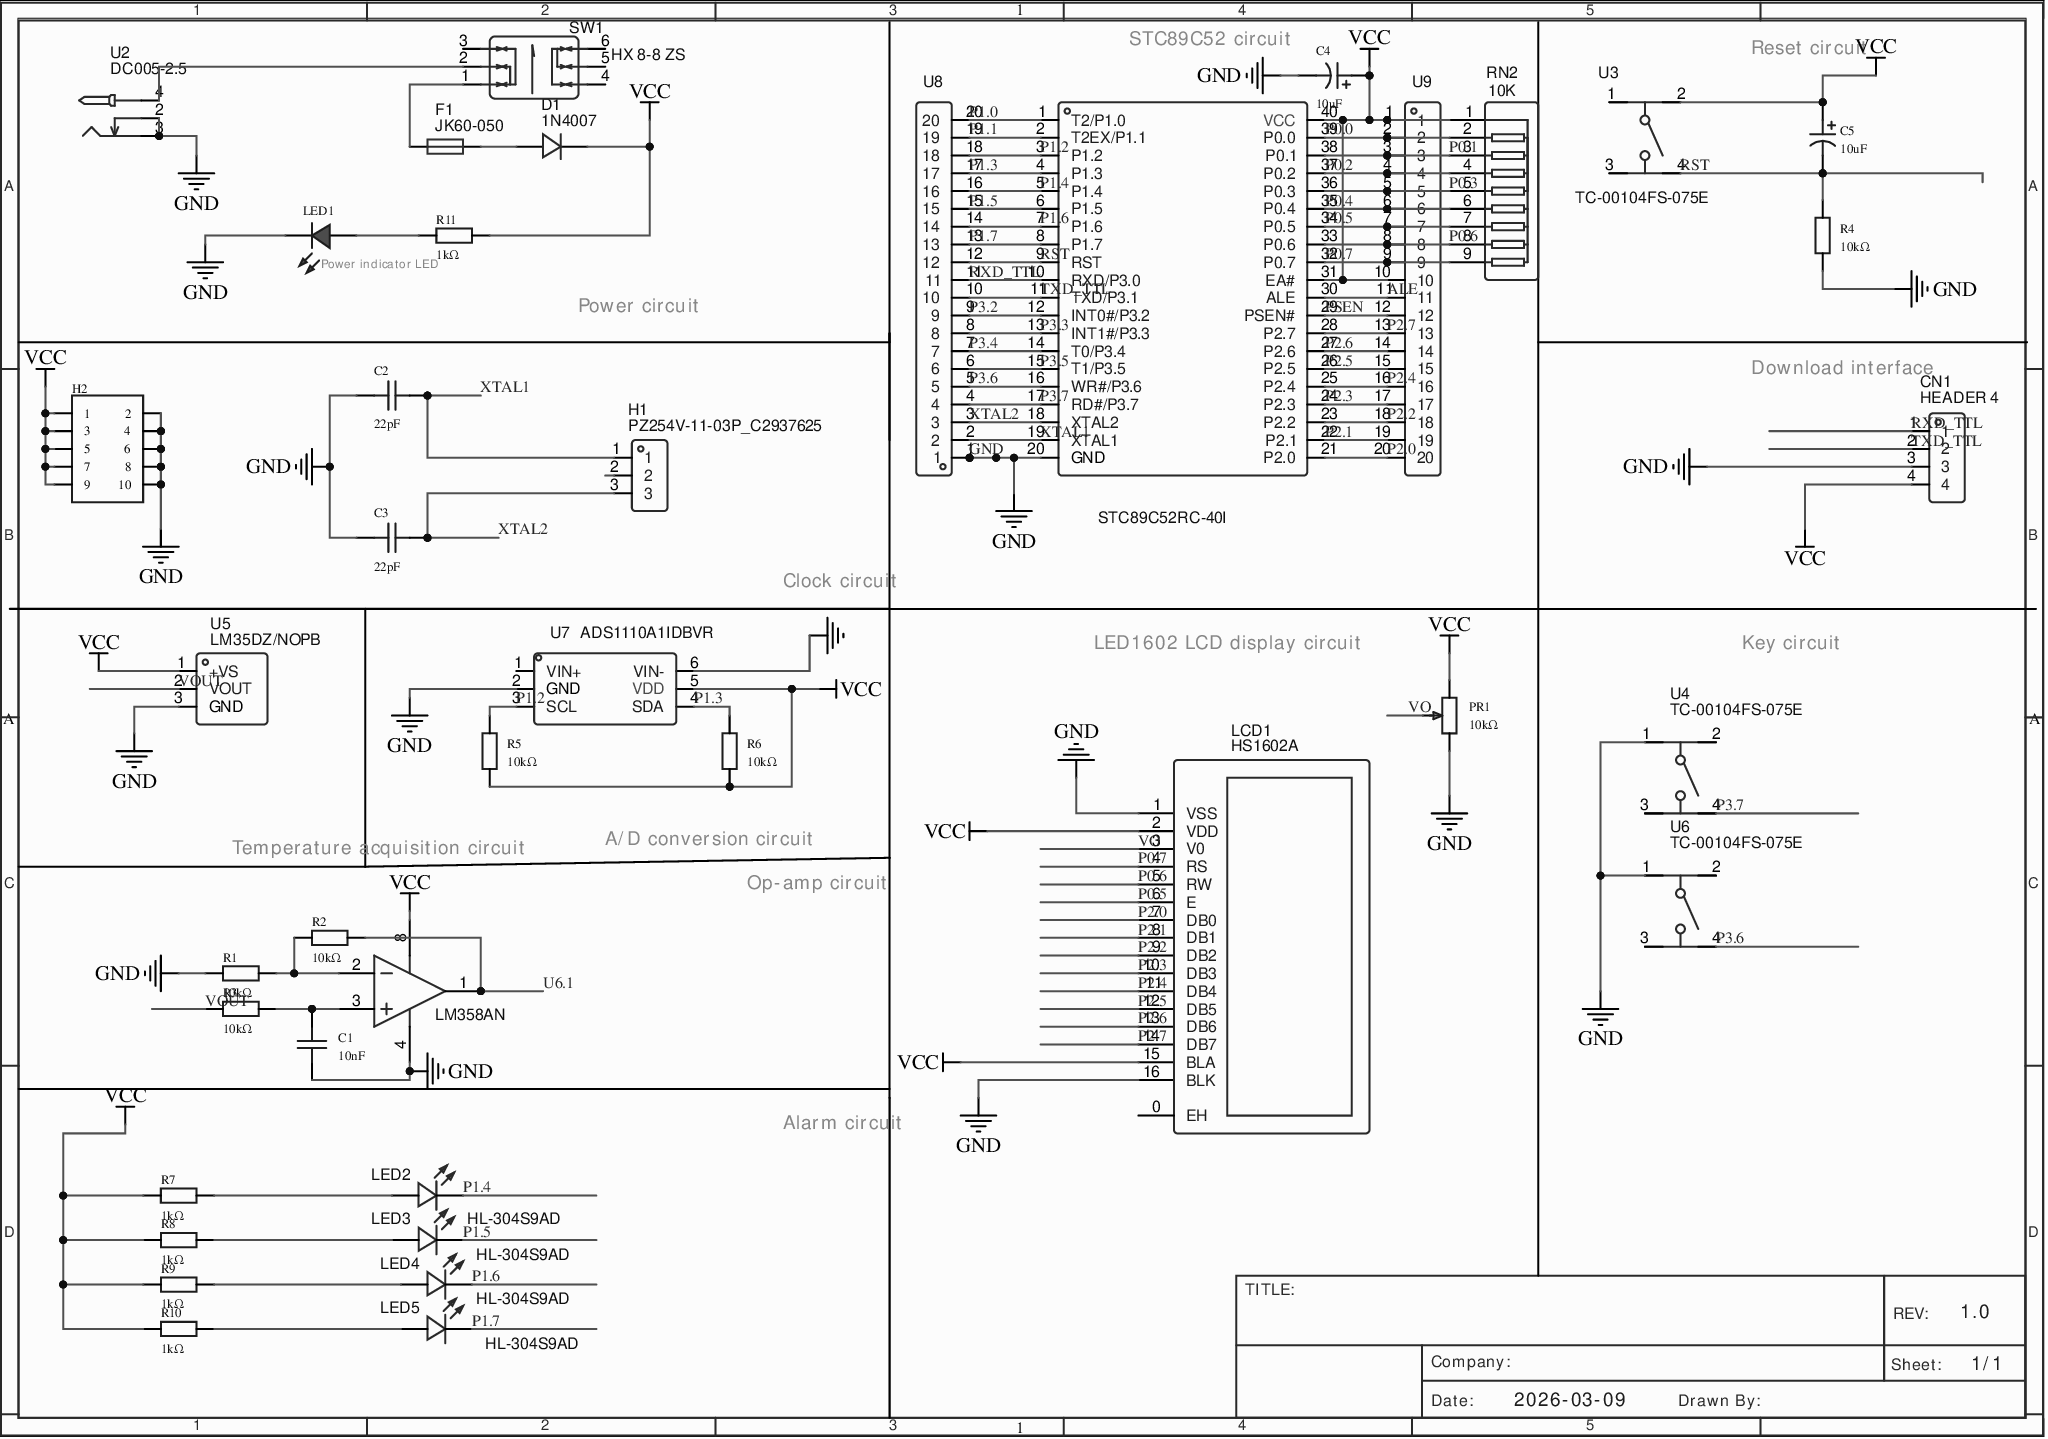
[diagram p0: MISC75226-3.schdoc]
# Altium project MISC75226-2.PrjPcb
1 sheet, 40 parts. Net scope: global (net labels, ports and power ports of the same name join across sheets).
Board file: MISC75226.pcbdoc

## Sheet MISC75226-3.schdoc
size 292 x 205 mm; Name: MISC75226; @Project Name: MISC75226; REV: 1.0; Date: 2026-03-09; Sheet: 1/1; Manufacturer Part: ?

### Parts
C1  10nF  [CAP-TH_L4.5-W2.5-P5.00-D0.5]
C2  22pF  [CAP-TH_L4.8-W3.2-P5.08-D0.5]
C3  22pF  [CAP-TH_L4.8-W3.2-P5.08-D0.5]
C4  10uF  [CAP-TH_BD5.0-P2.00-D0.8-FD-10UF50VC110GL]
C5  10uF  [CAP-TH_BD5.0-P2.00-D0.8-FD-10UF50VC110GL]
CN1  HEADER 4  [CONN-TH_XH-4A]
D1  1N4007  [DO-41_BD2.4-L4.7-P8.70-D0.9-RD]
F1  JK60-050  [FUSE-TH_L8.9-W3.0-P5.10-D0.6-S1.20]
H1  PZ254V-11-03P_C2937625  [HDR-TH_3P-P2.54-V-M_PZ254V-11-03P]
H2  (no value)  [HDR-TH_10P-P2.54-V-F-R2-C5-S2.54]
LCD1  HS1602A  [LCD1602]
LED1  (no value)  [LED_TH-3mm]
LED2  HL-304S9AD  [LED-TH_BD3.0-P2.54-FD]
LED3  HL-304S9AD  [LED-TH_BD3.0-P2.54-FD]
LED4  HL-304S9AD  [LED-TH_BD3.0-P2.54-FD]
LED5  HL-304S9AD  [LED-TH_BD3.0-P2.54-FD]
PR1  10kΩ  [R_3296]
R1  10kΩ  [Res_1/8W]
R2  10kΩ  [Res_1/8W]
R3  10kΩ  [Res_1/8W]
R4  10kΩ  [Res_1/8W]
R5  10kΩ  [Res_1/8W]
R6  10kΩ  [Res_1/8W]
R7  1kΩ  [Res_1/8W]
R8  1kΩ  [Res_1/8W]
R9  1kΩ  [Res_1/8W]
R10  1kΩ  [Res_1/8W]
R11  1kΩ  [Res_1/8W]
RN2  10K  [RES-ARRAY-TH_9P-P2.54-D1.0]
SW1  HX 8-8 ZS  [SW-TH_6P-L8.0-W8.0-P2.50-TL]
U1  LM358AN  [DIP-8_L9.8-W6.6-P2.54-LS7.6-BL]
U2  DC005-2.5  [DC-IN-TH_DC005-2.5MM]
U3  TC-00104FS-075E  [KEY-TH_4P-L6.0-W6.0-P4.50-LS6.5]
U4  TC-00104FS-075E  [KEY-TH_4P-L6.0-W6.0-P4.50-LS6.5]
U5  LM35DZ/NOPB  [TO-92-3_L4.8-W3.7-P2.54-L]
U6  TC-00104FS-075E  [KEY-TH_4P-L6.0-W6.0-P4.50-LS6.5]
U7  ADS1110A1IDBVR  [SOT-23-6_L2.9-W1.6-P0.95-LS2.8-BR]
U8  [Plugin] 2.54MM 1*20P straight female header-H5.0  [HDR-TH_20P-P2.54_C9900009338]  (value not drawn)
U9  [Plugin] 2.54MM 1*20P straight female header-H5.0  [HDR-TH_20P-P2.54_C9900009338]  (value not drawn)
U100  STC89C52RC-40I  [DIP-40_L52.0-W13.7-P2.54-LS15.2-BL]

### Nets
GND: C1.1 C2.1 C3.1 C4.2 CN1.3 H2.2 H2.4 H2.6 H2.8 H2.10 LCD1.1(VSS) LCD1.16(BLK) LED1.2(A) PR1.3 R1.1 R4.1 U1.4(GND) U2.2 U2.3 U4.1 U5.3(GND) U6.1 U7.2(GND) U7.6(VIN-) U8.1 U100.20(GND)
VCC: C4.1 C5.1 CN1.4 D1.1(K) H2.1 H2.3 H2.5 H2.7 H2.9 LCD1.2(VDD) LCD1.15(BLA) PR1.1 R5.1 R6.1 R7.1 R8.1 R9.1 R10.1 R11.2 RN2.1 U1.8(VCC) U3.2 U5.1(+VS) U7.5(VDD) U9.1 U9.10 U100.31(EA#) U100.40(VCC)
ALE: U9.11 U100.30(ALE)
P0.0: RN2.2 U9.2 U100.39(P0.0)
P0.1: RN2.3 U9.3 U100.38(P0.1)
P0.2: RN2.4 U9.4 U100.37(P0.2)
P0.3: RN2.5 U9.5 U100.36(P0.3)
P0.4: RN2.6 U9.6 U100.35(P0.4)
P0.5: LCD1.6(E) RN2.7 U9.7 U100.34(P0.5)
P0.6: LCD1.5(RW) RN2.8 U9.8 U100.33(P0.6)
P0.7: LCD1.4(RS) RN2.9 U9.9 U100.32(P0.7)
P1.0: U8.20 U100.1(T2/P1.0)
P1.1: U8.19 U100.2(T2EX/P1.1)
P1.2: R5.2 U7.3(SCL) U8.18 U100.3(P1.2)
P1.3: R6.2 U7.4(SDA) U8.17 U100.4(P1.3)
P1.4: LED2.2(C) U8.16 U100.5(P1.4)
P1.5: LED3.2(C) U8.15 U100.6(P1.5)
P1.6: LED4.2(C) U8.14 U100.7(P1.6)
P1.7: LED5.2(C) U8.13 U100.8(P1.7)
P2.0: LCD1.7(DB0) U9.20 U100.21(P2.0)
P2.1: LCD1.8(DB1) U9.19 U100.22(P2.1)
P2.2: LCD1.9(DB2) U9.18 U100.23(P2.2)
P2.3: LCD1.10(DB3) U9.17 U100.24(P2.3)
P2.4: LCD1.11(DB4) U9.16 U100.25(P2.4)
P2.5: LCD1.12(DB5) U9.15 U100.26(P2.5)
P2.6: LCD1.13(DB6) U9.14 U100.27(P2.6)
P2.7: LCD1.14(DB7) U9.13 U100.28(P2.7)
P3.2: U8.9 U100.12(INT0#/P3.2)
P3.3: U8.8 U100.13(INT1#/P3.3)
P3.4: U8.7 U100.14(T0/P3.4)
P3.5: U8.6 U100.15(T1/P3.5)
P3.6: U6.4 U8.5 U100.16(WR#/P3.6)
P3.7: U4.4 U8.4 U100.17(RD#/P3.7)
PSEN: U9.12 U100.29(PSEN#)
RST: C5.2 R4.2 U3.4 U8.12 U100.9(RST)
RXD_TTL: CN1.1 U8.11 U100.10(RXD/P3.0)
TXD_TTL: CN1.2 U8.10 U100.11(TXD/P3.1)
U6.1: R2.2 U1.1(OUT1)
VO: LCD1.3(V0) PR1.2
VOUT: R3.1 U5.2(VOUT)
XTAL1: C2.2 H1.1 U8.2 U100.19(XTAL1)
XTAL2: C3.2 H1.3 U8.3 U100.18(XTAL2)
NetC1_2: C1.2 R3.2 U1.3(IN1(+))
NetD1_2: D1.2(A) F1.2
NetF1_1: F1.1 SW1.1
NetLED1_1: LED1.1(C) R11.1
NetLED2_1: LED2.1(A) R7.2
NetLED3_1: LED3.1(A) R8.2
NetLED4_1: LED4.1(A) R9.2
NetLED5_1: LED5.1(A) R10.2
NetR1_2: R1.2 R2.1 U1.2(IN1(-))
NetSW1_2: SW1.2 U2.4

Not connected (* = marked no-connect by the designer): H1 2; LCD1 0(EH); SW1 3 4 5 6; U3 1 3; U4 2 3; U6 2 3; U7 1(VIN+)

### Notes on the sheet
- (near C4) STC89C52 circuit
- (near C5) Reset circuit
- Power indicator LED
- Power circuit
- (near CN1) Download interface
- Clock circuit
- LED1602 LCD display circuit
- Key circuit
- Temperature acquisition circuit
- (near R6) A/D conversion circuit
- Op-amp circuit
- Alarm circuit
- 1
- 2
- 3
- 4
- 5
- A
- B
- C
- D
- TITLE:
- Company:
- Sheet:
- REV:
- 1.0
- 1/1
- Date:
- 2026-03-09
- Drawn By:

### Library data of the parts
C1 = FK24C0G1H103JN006: 容值:10nF;精度:±5%;额定电压:50V;温度系数:C0G；NP0;; Manufacturer: TDK; AddInBom: yes; ModelId: a3610cc4d782423286e41c4ef8ce78f40819f05c4eef4c71ace90d822a990e87; ModelTransform: 216.535,98.8187,0,0,0,0,0,0,-196.85; Tolerance: ±5%; Voltage Rating: 50V; Temperature Coefficient: C0G; NP0; Symbol: FK24C0G1H103JN006; Device: FK24C0G1H103JN006; LCSC Part Name: 10nF ±5% 50V; SupplierPart: C5640246; ManufacturerPart: FK24C0G1H103JN006; Supplier Footprint: -; JLCPCB Part Class: Extended Part; Datasheet: https://item.szlcsc.com/datasheet/FK24C0G1H103JN006/6560964.html; Supplier: LCSC; ConvertToPcb: yes; FootprintName: CAP-TH_L4.5-W2.5-P5.00-D0.5; ModelName: CAP-TH_L4.5-W2.5-P5.00-D0.5; Value: 10nF
C2 C3 = CC4-0805-CG-50V-22pF-J: 容值:22pF;精度:±5%;额定电压:50V;温度系数:-;; Manufacturer: TORCH(火炬); AddInBom: yes; ModelId: f657e7819ee0481b9510acb89a450e410819f05c4eef4c71ace90d822a990e87; ModelName: CAP-TH_L4.8-W3.2-H6.8-P5.08; ModelTransform: 215.7476,125.984,0,0,0,0,0,0,-137.795; Tolerance: ±5%; Voltage Rating: 50V; Symbol: CC4-0805-CG -50V-22pF-J; Device: CC4-0805-CG-50V-22pF-J; LCSC Part Name: 22pF ±5% 50V; SupplierPart: C123150; ManufacturerPart: CC4-0805-CG-50V-22pF-J; Supplier Footprint: 插件,P=5.08mm; JLCPCB Part Class: Extended Part; Datasheet: https://item.szlcsc.com/datasheet/CC4-0805-CG-50V-22pF-J/124420.html; Supplier: LCSC; ConvertToPcb: yes; FootprintName: CAP-TH_L4.8-W3.2-P5.08-D0.5; Value: 22pF; Temperature Coefficient: -
C4 C5 = 10UF50VC110GL: 容值:10uF;精度:±20%;额定电压:50V;纹波电流:120mA@100KHz;等效串联电阻(ESR):1.6Ω;; Manufacturer: Econd(米朗电子); AddInBom: yes; Tolerance: ±20%; Voltage Rating: 50V; Equivalent Series Resistance(ESR): 1.6Ω; Pin Spacing: 2mm; Lifetime: 5000hrs@105℃; Symbol: 10UF50VC110GL; Device: 10UF50VC110GL; LCSC Part Name: 10uF ±20% 50V; SupplierPart: C46867109; ManufacturerPart: 10UF50VC110GL; Supplier Footprint: 插件,D5xL11mm; JLCPCB Part Class: Extended Part; Datasheet: https://item.szlcsc.com/datasheet/10UF50VC110GL/49031974.html; Supplier: LCSC; ConvertToPcb: yes; FootprintName: CAP-TH_BD5.0-P2.00-D0.8-FD-10UF50VC110GL; Value: 10uF; Ripple Current: 120mA@100KHz; Diameter: 5mm; Height - Seated (Max): 11mm; Operating Temperature: -40℃~+105℃
CN1 = Header 4: Manufacturer: null; Convert to PCB: yes; UniqueId: ggea3fdb8c5cd09fd78; ModelTransform: 492.125,228.346,0,0,0,0,-0.003,20.196,-129.921; Device: Header 4; Supplier: LCSC; Supplier Part: C9900017655; Manufacturer Part: Header 4; JLCPCB Part Class: Extended Part; Add into BOM: yes; SymbolName: HEADER 4; FootprintName: CONN-TH_XH-4A; OriginModelName: CONN-TH_XH-4A
D1 = 1N4007: Manufacturer: ST(先科); Convert to PCB: yes; UniqueId: ggea25f4b96c0c873f1; OriginModelName: DO-41_D2.4-L4.7-P8.70; ModelTransform: 374.016,94.488,0,0,0,0,0.002,0,-137.795; Device: 1N4007; Supplier: LCSC; Manufacturer Part: 1N4007; Supplier Part: C106903; JLCPCB Part Class: Extended Part; Add into BOM: yes; SymbolName: 1N4007; FootprintName: DO-41_BD2.4-L4.7-P8.70-D0.9-RD
F1 = JK60-050: Manufacturer: null; Convert to PCB: yes; UniqueId: gge1ed7edf1a1e32f02; OriginModelName: FUSE-TH_L8.9-W3.0-H13.5-P5.1-D0.6-S1.2; ModelTransform: 350.393,118.11,0,0,0,0,0,0,-275.591; Device: JK60-050; Supplier: LCSC; Supplier Part: C139092; Manufacturer Part: JK60-050; JLCPCB Part Class: Extended Part; Add into BOM: yes; SymbolName: JK60-050; FootprintName: FUSE-TH_L8.9-W3.0-P5.10-D0.6-S1.20
H1 = PZ254V-11-03P: Manufacturer: XFCN(兴飞); Convert to PCB: yes; UniqueId: ggee8450ff7c7c91b07; ModelTransform: 300.3931,100,0,0,0,0,-0.001,0.001,-118.11; Device: PZ254V-11-03P; Supplier: LCSC; Supplier Part: C2937625; Manufacturer Part: PZ254V-11-03P; JLCPCB Part Class: Extended Part; Add into BOM: yes; SymbolName: PZ254V-11-03P_C2937625; FootprintName: HDR-TH_3P-P2.54-V-M_PZ254V-11-03P; OriginModelName: HDR-TH_3P-P2.54-V-M_PZ254V-11-03P
H2 = HDR-F_2.54_2x5: Symbol: HDR-F-2.54_2x5; ConvertToPcb: yes; ModelId: 86e5d65f54dd476391caab3fdb9168240819f05c4eef4c71ace90d822a990e87; ModelName: HDR2.54-F-LI-2X5P; ModelTransform: 499.999,200,0,0,0,0,0,0,-118.11; Device: HDR-F_2.54_2x5; AddInBom: yes; SupplierPart: C92270; Supplier Footprint: 插件; FootprintName: HDR-TH_10P-P2.54-V-F-R2-C5-S2.54
LCD1 = HS1602A: Manufacturer: HS(汉昇); Convert to PCB: yes; UniqueId: gge471e28896b9a3d54; ModelTransform: 3149.6,1417.32,0,0,0,0,0,0,-118.11; Device: HS1602A; Supplier: LCSC; Supplier Part: C5329588; Manufacturer Part: HS1602A; JLCPCB Part Class: Extended Part; Add into BOM: yes; SymbolName: HS1602A; FootprintName: LCD1602; OriginModelName: LCD1602
LED1 = LED_TH-R_3mm: ConvertToPcb: yes; ModelId: a497c992633541038a38947cdc58012f0819f05c4eef4c71ace90d822a990e87; ModelName: LED-TH-3mm_R; ModelTransform: 141.274,153.327,0,0,0,0,-5.984,0,-137.795; Symbol: LED_TH-R; Device: LED_TH-R_3mm; AddInBom: yes; FootprintName: LED_TH-3mm; Supplier Footprint: 插件
LED2 = HL-304S9AD: Manufacturer: HONGLITRONIC(鸿利光电); Convert to PCB: yes; UniqueId: ggedcb368d0afbaf50c; OriginModelName: LED-TH-3mm_R; ModelTransform: 141.274,153.327,0,0,0,0,-5.983,0,-137.795; Device: HL-304S9AD; Supplier: LCSC; Supplier Part: C568936; Manufacturer Part: HL-304S9AD; JLCPCB Part Class: Extended Part; Add into BOM: yes; SymbolName: HL-304S9AD; FootprintName: LED-TH_BD3.0-P2.54-FD
LED3 = HL-304S9AD: Manufacturer: HONGLITRONIC(鸿利光电); Convert to PCB: yes; UniqueId: gge7e573e1ae17299c8; OriginModelName: LED-TH-3mm_R; ModelTransform: 141.274,153.327,0,0,0,0,-5.983,0,-137.795; Device: HL-304S9AD; Supplier: LCSC; Supplier Part: C568936; Manufacturer Part: HL-304S9AD; JLCPCB Part Class: Extended Part; Add into BOM: yes; SymbolName: HL-304S9AD; FootprintName: LED-TH_BD3.0-P2.54-FD
LED4 = HL-304S9AD: Manufacturer: HONGLITRONIC(鸿利光电); Convert to PCB: yes; UniqueId: gge9c2f58a485d7e2d3; OriginModelName: LED-TH-3mm_R; ModelTransform: 141.274,153.327,0,0,0,0,-5.983,0,-137.795; Device: HL-304S9AD; Supplier: LCSC; Supplier Part: C568936; Manufacturer Part: HL-304S9AD; JLCPCB Part Class: Extended Part; Add into BOM: yes; SymbolName: HL-304S9AD; FootprintName: LED-TH_BD3.0-P2.54-FD
LED5 = HL-304S9AD: Manufacturer: HONGLITRONIC(鸿利光电); Convert to PCB: yes; UniqueId: ggec88dd7fe630cf856; OriginModelName: LED-TH-3mm_R; ModelTransform: 141.274,153.327,0,0,0,0,-5.983,0,-137.795; Device: HL-304S9AD; Supplier: LCSC; Supplier Part: C568936; Manufacturer Part: HL-304S9AD; JLCPCB Part Class: Extended Part; Add into BOM: yes; SymbolName: HL-304S9AD; FootprintName: LED-TH_BD3.0-P2.54-FD
PR1 = R_3296: ConvertToPcb: yes; ModelId: b182808559bb43bda9e7de64b64134cb0819f05c4eef4c71ace90d822a990e87; ModelName: 3296W; ModelTransform: 373.98,188.96,590.49,180,0,0,0,0,-140; Symbol: R_3296; Device: R_3296; AddInBom: yes; Supplier Footprint: 直插; FootprintName: R_3296; Value: 10kΩ
R1-R11 = Res_AXIAL-1/8W: Symbol: Resistor; ConvertToPcb: yes; ModelId: b2b5ae7ae4c642178fe0039925c86a3f0819f05c4eef4c71ace90d822a990e87; ModelName: RES-TH_BD1.8-L3.2-P7.20-D0.4; ModelTransform: 282.86,66.88,253.09,0,0,0,0,0,-191; Device: Res_AXIAL-1/8W; AddInBom: yes; Supplier Footprint: 轴向引线; FootprintName: Res_1/8W
  R1-R6: Value: 10kΩ
  R7-R11: Value: 1kΩ
RN2 = 排阻 10 K 5%: Manufacturer: null; Device: Resistor array 10 K 5%; Convert to PCB: yes; UniqueId: ggeefe6aabb381e25da; OriginModelName: SIP-9_L22.8-W3.0-H8.5-P2.54; ModelTransform: 917.49722,118.11,0,0,0,0,-0.001,0,-137.795; Supplier: LCSC; Manufacturer Part: 排阻 10 K 5%; Supplier Part: C26615; JLCPCB Part Class: Extended Part; Add into BOM: yes; SymbolName: 10K; FootprintName: RES-ARRAY-TH_9P-P2.54-D1.0
SW1 = HX 8-8 ZS: Manufacturer: hanxia(韩下); Convert to PCB: yes; UniqueId: gge535e4f6a2a2525e2; ModelTransform: 314.96394,314.96,0,90,0,0,-0.002,0,-137.795; Device: HX 8-8 ZS; Supplier: LCSC; Supplier Part: C7435563; Manufacturer Part: HX 8-8 ZS; JLCPCB Part Class: Extended Part; Add into BOM: yes; SymbolName: HX 8-8 ZS; FootprintName: SW-TH_6P-L8.0-W8.0-P2.50-TL; OriginModelName: SW-TH_6P-L8.0-W8.0-P2.50-TL
U1 = LM358AN: Manufacturer: onsemi(安森美); Convert to PCB: yes; UniqueId: ggec840bfe444e1d986; OriginModelName: DIP-8_L9.8-W6.6-H3.5-LS7.62-P2.54; ModelTransform: 385.826,311.8104,0,0,0,0,-1.693,-0.002,-137.795; Device: LM358AN; Supplier: LCSC; Manufacturer Part: LM358AN; Supplier Part: C95623; JLCPCB Part Class: Extended Part; Add into BOM: yes; SymbolName: LM358AN; FootprintName: DIP-8_L9.8-W6.6-P2.54-LS7.6-BL
U2 = DC005-2.5: Manufacturer: SHOU HAN(首韩); Convert to PCB: yes; UniqueId: ggefa72b7768d961f25; ModelTransform: 559.054,366.18037,0,0,0,0,-139.178,86.971,-157.48; Device: DC005-2.5; Supplier: LCSC; Supplier Part: C7507454; Manufacturer Part: DC005-2.5; JLCPCB Part Class: Extended Part; Add into BOM: yes; SymbolName: DC005-2.5; FootprintName: DC-IN-TH_DC005-2.5MM; OriginModelName: DC-IN-TH_DC005-2.5MM
U3 = TC-00104FS-075E: Manufacturer: HOOYA(皓宇电子); Convert to PCB: yes; UniqueId: gge10e57302bf5a9b7a; ModelTransform: 236.25937,323.03,0,90,0,0,-0.001,-0.001,-137.795; Device: TC-00104FS-075E; Supplier: LCSC; Supplier Part: C4355198; Manufacturer Part: TC-00104FS-075E; JLCPCB Part Class: Extended Part; Add into BOM: yes; SymbolName: TC-00104FS-075E; FootprintName: KEY-TH_4P-L6.0-W6.0-P4.50-LS6.5; OriginModelName: KEY-TH_4P-L6.0-W6.0-P4.50-LS6.5
U4 = TC-00104FS-075E: Manufacturer: HOOYA(皓宇电子); Convert to PCB: yes; UniqueId: gge9f30e894b082ac1c; ModelTransform: 236.25937,323.03,0,90,0,0,-0.001,-0.001,-137.795; Device: TC-00104FS-075E; Supplier: LCSC; Supplier Part: C4355198; Manufacturer Part: TC-00104FS-075E; JLCPCB Part Class: Extended Part; Add into BOM: yes; SymbolName: TC-00104FS-075E; FootprintName: KEY-TH_4P-L6.0-W6.0-P4.50-LS6.5; OriginModelName: KEY-TH_4P-L6.0-W6.0-P4.50-LS6.5
U5 = LM35DZ/NOPB: Manufacturer: null; Convert to PCB: yes; UniqueId: gge29105a6ecc7d3b00; OriginModelName: TO-92-3_L4.8-W3.7-H4.8-P2.54; ModelTransform: 218.1098,145.669,0,0,0,0,0,13.779,-137.795; Device: LM35DZ/NOPB; Supplier: LCSC; Supplier Part: C363277; Manufacturer Part: LM35DZ/NOPB; JLCPCB Part Class: Extended Part; Add into BOM: yes; SymbolName: LM35DZ/NOPB; FootprintName: TO-92-3_L4.8-W3.7-P2.54-L
U6 = TC-00104FS-075E: Manufacturer: HOOYA(皓宇电子); Convert to PCB: yes; UniqueId: gge522915879370b8c0; ModelTransform: 236.25937,323.03,0,90,0,0,-0.001,-0.001,-137.795; Device: TC-00104FS-075E; Supplier: LCSC; Supplier Part: C4355198; Manufacturer Part: TC-00104FS-075E; JLCPCB Part Class: Extended Part; Add into BOM: yes; SymbolName: TC-00104FS-075E; FootprintName: KEY-TH_4P-L6.0-W6.0-P4.50-LS6.5; OriginModelName: KEY-TH_4P-L6.0-W6.0-P4.50-LS6.5
U7 = ADS1110A1IDBVR: Manufacturer: TI(德州仪器); Convert to PCB: yes; UniqueId: gge42ce37e384c9c669; OriginModelName: SOT-23-6_L2.9-W1.6-H1.5-LS2.8-P0.95; ModelTransform: 110.73671,114.173,0,180,0,0,0.001,-0.003,0; Device: ADS1110A1IDBVR; Supplier: LCSC; Supplier Part: C2670231; Manufacturer Part: ADS1110A1IDBVR; JLCPCB Part Class: Extended Part; Add into BOM: yes; SymbolName: ADS1110A1IDBVR; FootprintName: SOT-23-6_L2.9-W1.6-P0.95-LS2.8-BR
U8 = [插件] 2.54mm 1*20P 直排母-H5.0: Manufacturer: null; Convert to PCB: yes; UniqueId: gge4b7f33523c12f523; ModelTransform: 1999.996,110.236,0,0,0,0,0.001,0,-122.047; Device: [Plugin] 2.54mm 1*20P straight female header-H5.0; Supplier: LCSC; Supplier Part: C9900009338; Manufacturer Part: [插件] 2.54mm 1*20P 直排母-H5.0; JLCPCB Part Class: Extended Part; Add into BOM: yes; SymbolName: [Plugin] 2.54MM 1*20P straight female header-H5.0; FootprintName: HDR-TH_20P-P2.54_C9900009338; OriginModelName: HDR-TH_20P-P2.54_C9900009338
U9 = [插件] 2.54mm 1*20P 直排母-H5.0: Manufacturer: null; Convert to PCB: yes; UniqueId: ggec78c4102e6db526a; ModelTransform: 1999.996,110.236,0,0,0,0,0.001,0,-122.047; Device: [Plugin] 2.54mm 1*20P straight female header-H5.0; Supplier: LCSC; Supplier Part: C9900009338; Manufacturer Part: [插件] 2.54mm 1*20P 直排母-H5.0; JLCPCB Part Class: Extended Part; Add into BOM: yes; SymbolName: [Plugin] 2.54MM 1*20P straight female header-H5.0; FootprintName: HDR-TH_20P-P2.54_C9900009338; OriginModelName: HDR-TH_20P-P2.54_C9900009338
U100 = STC89C52RC-40I-PDIP40: Manufacturer: STC; Convert to PCB: yes; UniqueId: ggef9540a4f372c878e; OriginModelName: DIP-40_L52.3-W13.8-H4.0-LS15.24-P2.54; ModelTransform: 2059.051,615.743,0,0,0,0,0.001,0,-118.11; Device: STC89C52RC-40I-PDIP40; Supplier: LCSC; Manufacturer Part: STC89C52RC-40I-PDIP40; Supplier Part: C14022; JLCPCB Part Class: Extended Part; Add into BOM: yes; SymbolName: STC89C52RC-40I; FootprintName: DIP-40_L52.0-W13.7-P2.54-LS15.2-BL